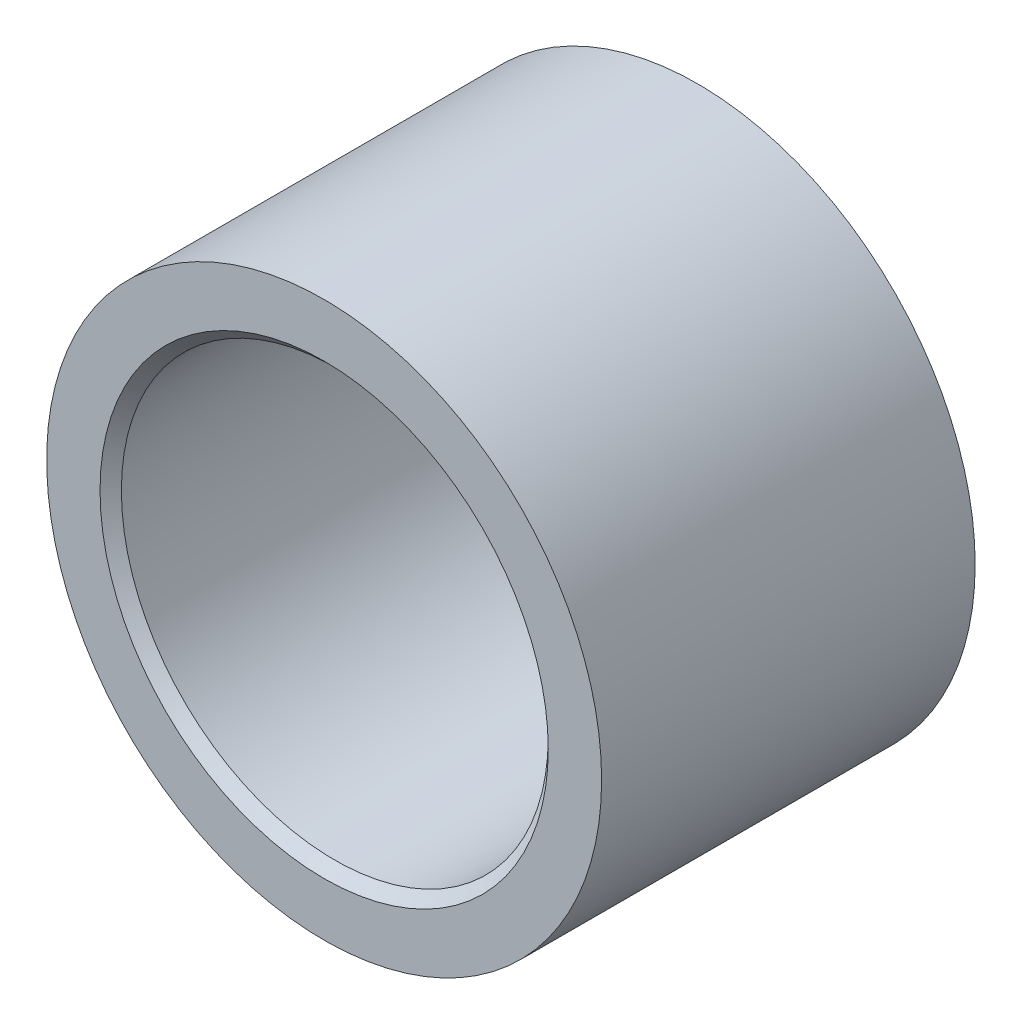
from build123d import *

# Parameters (mm, degrees)
SKETCH1_R           = 13
SKETCH1_R_2         = 10
BOSS_EXTRUDE1_DEPTH = 17.5
CHAMFER1_SIZE       = 0.5


with BuildPart() as part:
    # Sketch1 → Boss-Extrude1 (new body)
    with BuildSketch(Plane.XY):
        Circle(SKETCH1_R)
        Circle(SKETCH1_R_2, mode=Mode.SUBTRACT)
    extrude(amount=BOSS_EXTRUDE1_DEPTH)

    # Chamfer1
    chamfer1_edges = [part.edges().sort_by_distance(p)[0] for p in [
        (-10, 0, 0),
        (-10, 0, 17.5),
    ]]
    chamfer(chamfer1_edges, length=CHAMFER1_SIZE)


solid = part.part
